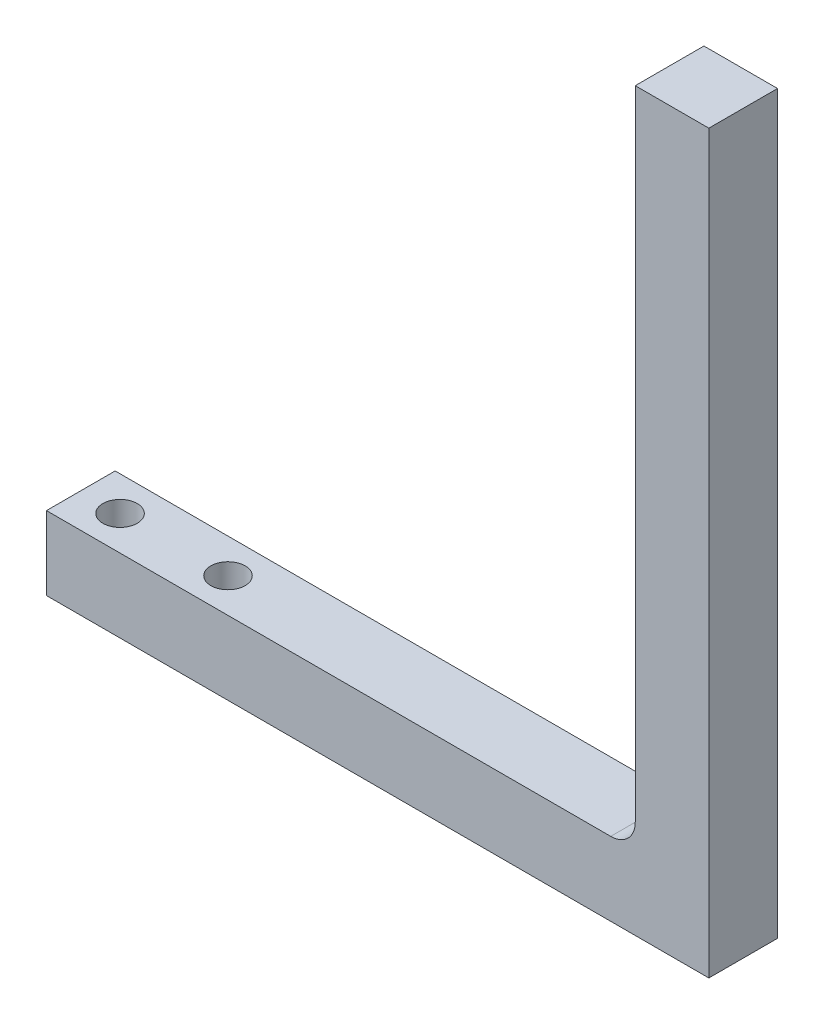
from build123d import *

# Parameters (mm, degrees)
EXTRUDE_1_DEPTH     = 7
FILLET_1_R          = 5
CUT_EXTRUDE_1_REACH = 193.047
SKETCH_3_R          = 3.5


with BuildPart() as part:
    # 草图1 → 凸台-拉伸1 (new, symmetric)
    with BuildSketch(Plane.XY):
        Polygon((0, 150), (-15, 150), (-15, 15), (-135, 15), (-135, 0), (0, 0), align=None)
    extrude(amount=EXTRUDE_1_DEPTH, both=True)

    # 圆角1
    fillet_1_edges = [part.edges().sort_by_distance(p)[0] for p in [
        (-15, 15, 0),
    ]]
    fillet(fillet_1_edges, radius=FILLET_1_R)

    # 草图3 → 切除-拉伸1 (cut, up to next)
    with BuildSketch(Plane(origin=(0, 15, 0), x_dir=(1, 0, 0), z_dir=(0, 1, 0)), mode=Mode.PRIVATE) as cut_extrude_1_sk1:
        with Locations(Location((-127, 0, 0), (0, 0, 180))):
            Circle(SKETCH_3_R)
    cut_extrude_1_tool1 = extrude(cut_extrude_1_sk1.sketch, amount=-CUT_EXTRUDE_1_REACH, mode=Mode.PRIVATE) & part.part
    # 草图3 → 切除-拉伸1 (cut, up to next)
    with BuildSketch(Plane(origin=(0, 15, 0), x_dir=(1, 0, 0), z_dir=(0, 1, 0)), mode=Mode.PRIVATE) as cut_extrude_1_sk2:
        with Locations(Location((-105, 0, 0), (0, 0, 180))):
            Circle(SKETCH_3_R)
    cut_extrude_1_tool2 = extrude(cut_extrude_1_sk2.sketch, amount=-CUT_EXTRUDE_1_REACH, mode=Mode.PRIVATE) & part.part
    add(cut_extrude_1_tool1.solids().sort_by_distance((-127, 15, 0))[0], mode=Mode.SUBTRACT)
    add(cut_extrude_1_tool2.solids().sort_by_distance((-105, 15, 0))[0], mode=Mode.SUBTRACT)


solid = part.part
